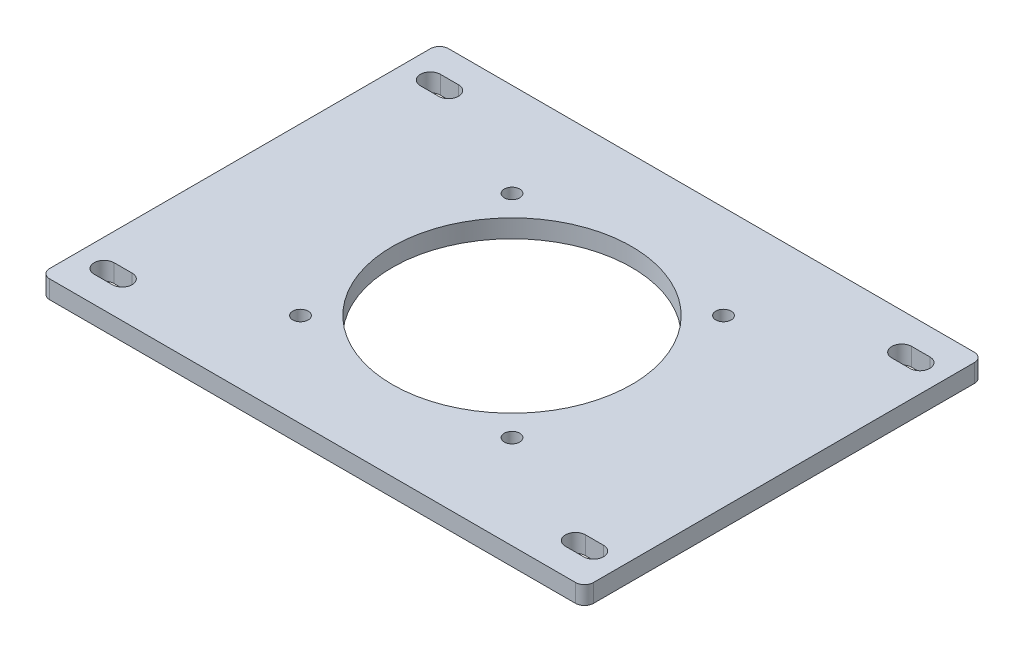
SolidWorks part; units mm, degrees
material "Q235"
ref_plane "Front Plane" through (0, 0, 0) normal (0, 0, 1) x (1, 0, 0)
ref_plane "Top Plane" through (0, 0, 0) normal (0, 1, 0) x (1, 0, 0)
ref_plane "Right Plane" through (0, 0, 0) normal (1, 0, 0) x (0, 0, -1)
sketch "Sketch1" plane through (0, 0, 0) normal (0, 1, 0) x (1, 0, 0)
  line L1 (-150, 110) -> (150, 110)
  line L2 (-150, 110) -> (-150, -110)
  line L3 (-150, -110) -> (150, -110)
  line L4 (150, 110) -> (150, -110)
  line L5 (-150, 110) -> (150, -110) construction
  line L6 (-150, -110) -> (150, 110) construction
  point P0 (0, 0)
  dimension "D1" = 220
  dimension "D2" = 300
extrude "Boss-Extrude1" add sketch "Sketch1" along normal blind 10
sketch "Sketch3" plane through (0, 10, 0) normal (0, 1, 0) x (1, 0, 0)
  circle A0 centre (0, 0) radius 66
  dimension "D1" = 132
extrude "Cut-Extrude1" cut sketch "Sketch3" against normal through all
hole_wizard "M10 Tapped Hole1" positions "Sketch4" profile "Sketch5" tap size "M10" standard "GB"
sketch "Sketch4" plane through (0, 10, 0) normal (0, 1, 0) x (1, 0, 0)
  line L0 (-58.3363, 58.3363) -> (58.3363, 58.3363) construction
  line L1 (58.3363, 58.3363) -> (58.3363, -58.3363) construction
  line L2 (58.3363, -58.3363) -> (-58.3363, -58.3363) construction
  circle A0 centre (0, 0) radius 82.5
  point P5 (-58.3363, 58.3363)
  point P7 (58.3363, 58.3363)
  point P9 (58.3363, -58.3363)
  point P11 (-58.3363, -58.3363)
  dimension "D1" = 165
sketch "Sketch5" plane through (-58.3363, 10, 58.3363) normal (1, 0, 0) x (0, 0, 1)
  line L0 (0, 0) -> (0, 27.0537)
  line L1 (0, 27.0537) -> (4.25, 24.5)
  line L2 (4.25, 24.5) -> (4.25, 0)
  line L5 (4.25, 0) -> (0, 0)
  line L10 (0, 27.0537) -> (-4.25, 24.5) construction
  line L11 (0, -6.35) -> (0, 107.95) construction
  dimension "螺纹孔钻头直径" = 8.5
  dimension "螺纹孔钻头深度" = 24.5
  dimension "导头角度" = 118
cosmetic thread "Cosmetic Thread1" parameters "D1"=8, "D2"=10
cosmetic thread "Cosmetic Thread2" parameters "D1"=8, "D2"=10
cosmetic thread "Cosmetic Thread3" parameters "D1"=8, "D2"=10
cosmetic thread "Cosmetic Thread4" parameters "D1"=8, "D2"=10
sketch "Sketch6" plane through (0, 10, 0) normal (0, 1, 0) x (1, 0, 0)
  line L0 (-135, 90) -> (-125, 90) construction
  line L1 (-135, 95.5) -> (-125, 95.5)
  line L2 (-135, 84.5) -> (-125, 84.5)
  line L3 (0, 110) -> (0, 85.2975) construction
  line L4 (150, 110) -> (-150, 110) construction
  line L5 (135, 90) -> (125, 90) construction
  line L6 (135, 95.5) -> (125, 95.5)
  line L7 (135, 84.5) -> (125, 84.5)
  line L8 (-150, 0) -> (-128.3388, 0) construction
  line L9 (-150, 110) -> (-150, -110) construction
  line L10 (135, -90) -> (125, -90) construction
  line L11 (135, -95.5) -> (125, -95.5)
  line L12 (135, -84.5) -> (125, -84.5)
  line L13 (-135, -90) -> (-125, -90) construction
  line L14 (-135, -95.5) -> (-125, -95.5)
  line L15 (-135, -84.5) -> (-125, -84.5)
  arc A0 (-135, 95.5) -> (-135, 84.5) centre (-135, 90) ccw
  arc A1 (-125, 84.5) -> (-125, 95.5) centre (-125, 90) ccw
  arc A2 (135, 95.5) -> (135, 84.5) centre (135, 90) cw
  arc A3 (125, 84.5) -> (125, 95.5) centre (125, 90) cw
  arc A4 (135, -95.5) -> (135, -84.5) centre (135, -90) ccw
  arc A5 (125, -84.5) -> (125, -95.5) centre (125, -90) ccw
  arc A6 (-135, -95.5) -> (-135, -84.5) centre (-135, -90) cw
  arc A7 (-125, -84.5) -> (-125, -95.5) centre (-125, -90) cw
  point P2 (-130, 90)
  point P14 (130, 90)
  point P25 (130, -90)
  point P32 (-130, -90)
  dimension "D4" = 180
  dimension "D1" = 11
  dimension "D2" = 260
  dimension "D3" = 10
extrude "Cut-Extrude2" cut sketch "Sketch6" against normal through all
fillet "Fillet1" radius 5 4 edges at (150, 5, 110) (150, 5, -110) (-150, 5, -110) (-150, 5, 110)
